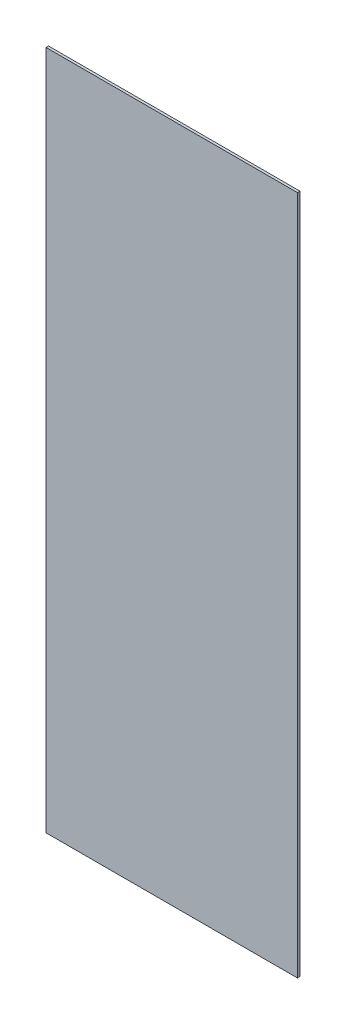
SolidWorks part; units mm, degrees
material "PMMA(有机玻璃)"
ref_plane "前视" through (0, 0, 0) normal (0, 0, 1) x (1, 0, 0)
ref_plane "上视" through (0, 0, 0) normal (0, 1, 0) x (1, 0, 0)
ref_plane "右视" through (0, 0, 0) normal (1, 0, 0) x (0, 0, -1)
sketch "草图1" plane through (0, 0, 0) normal (0, 0, 1) x (1, 0, 0)
  line L1 (-249.5, 675) -> (249.5, 675)
  line L2 (-249.5, 675) -> (-249.5, -675)
  line L3 (-249.5, -675) -> (249.5, -675)
  line L4 (249.5, 675) -> (249.5, -675)
  line L5 (-249.5, 675) -> (249.5, -675) construction
  line L6 (-249.5, -675) -> (249.5, 675) construction
  point P0 (0, 0)
  dimension "D1" = 1350
  dimension "D2" = 499
extrude "凸台-拉伸1" add sketch "草图1" along normal blind 5
hole_wizard "M5 间隙孔1" positions "草图3" profile "草图2" hole size "M5" standard "GB"
sketch "草图3" plane through (0, 0, 5) normal (0, 0, 1) x (1, 0, 0)
  line L0 (-427.5, 273) -> (-427.5, -273) construction
  line L1 (-427.5, -273) -> (427.5, -273) construction
  line L2 (0, 273) -> (0, -273) construction
  line L3 (427.5, 273) -> (-427.5, 273) construction
  line L5 (-427.5, 0) -> (427.5, 0) construction
  line L6 (427.5, -273) -> (427.5, 273) construction
  point P0 (-375, -261)
  point P46 (415.5, 250)
  point P48 (-415.5, 250)
  point P58 (-125, -261)
  point P59 (125, -261)
  point P61 (-125, 261)
  point P62 (125, 261)
  point P64 (-375, 261)
  point P88 (375, -261)
  point P89 (375, 261)
  point P108 (415.5, 0)
  point P109 (-415.5, 0)
  point P110 (415.5, -250)
  point P111 (-415.5, -250)
  dimension "D1" = 12
  dimension "D2" = 12
  dimension "D5" = 3
  dimension "D3" = 12
  dimension "D6" = 4
  dimension "D4" = 2
sketch "草图2" plane through (-375, -261, 5) normal (1, 0, 0) x (0, -1, 0)
  line L0 (0, 0) -> (0, 5)
  line L1 (0, 5) -> (2.75, 5)
  line L2 (2.75, 5) -> (2.75, 0)
  line L5 (2.75, 0) -> (0, 0)
  line L11 (0, -6.35) -> (0, 107.95) construction
  dimension "通孔孔直径" = 5.5
  dimension "通孔孔深度" = 5
